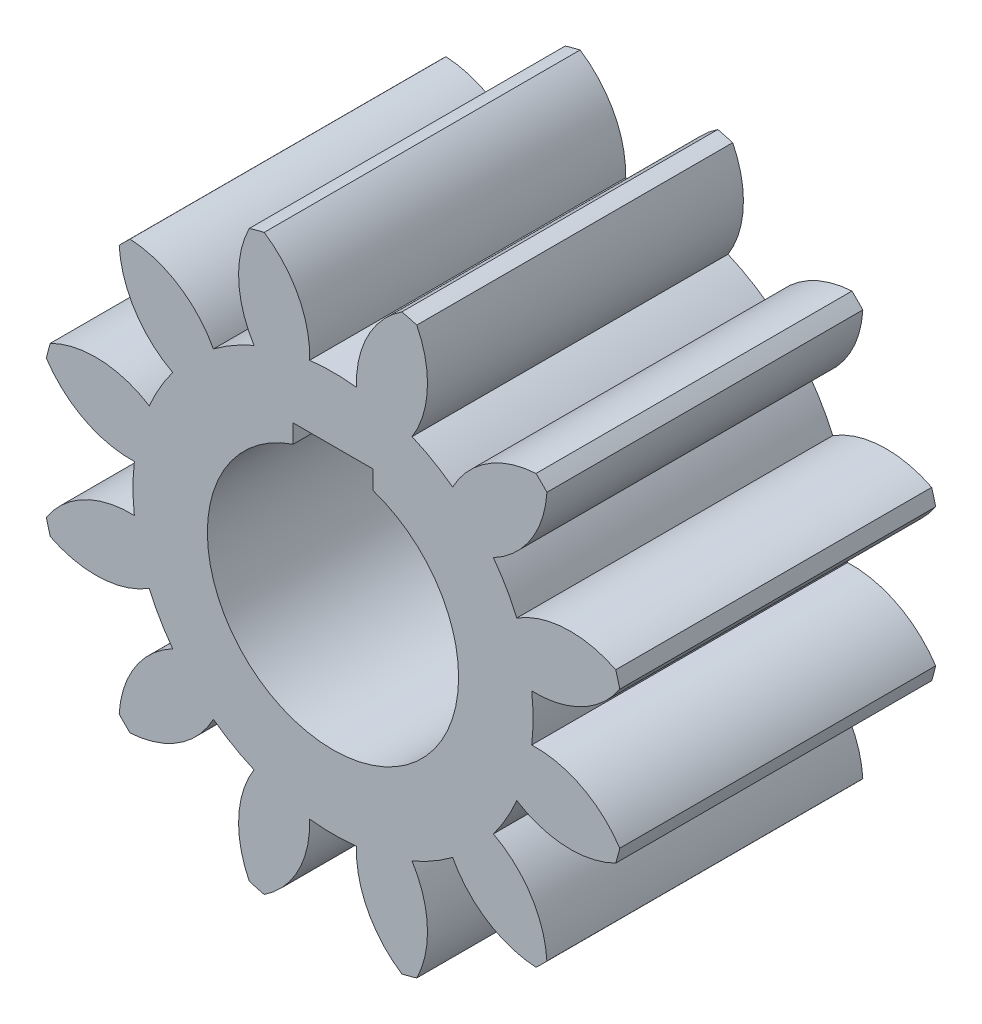
from build123d import *

# Parameters (mm, degrees)
EXTRUDE_1_DEPTH = 15


with BuildPart() as part:
    # 草图2 → 凸台-拉伸1 (new body)
    with BuildSketch(Plane.XY):
        with BuildLine():
            ThreePointArc((-10.154744655, 9.637487276), (-9.402240771, 7.326120193), (-7.613867765, 5.67979037))
            ThreePointArc((-7.613867765, 5.67979037), (-8.226375311, 4.7495), (-8.725776632, 3.753907721))
            ThreePointArc((-8.725776632, 3.753907721), (-11.045726583, 4.479519264), (-13.423681137, 3.975523202))
            ThreePointArc((-13.423681137, 3.975523202), (-13.522961568, 3.623466631), (-13.613010478, 3.268936482))
            ThreePointArc((-13.613010478, 3.268936482), (-11.805639456, 1.643485813), (-9.433698091, 1.111908866))
            ThreePointArc((-9.433698091, 1.111908866), (-9.499, 0), (-9.433698091, -1.111908866))
            ThreePointArc((-9.433698091, -1.111908866), (-11.805639456, -1.643485813), (-13.613010478, -3.268936482))
            ThreePointArc((-13.613010478, -3.268936482), (-13.522961568, -3.623466631), (-13.423681137, -3.975523202))
            ThreePointArc((-13.423681137, -3.975523202), (-11.045726583, -4.479519264), (-8.725776632, -3.753907721))
            ThreePointArc((-8.725776632, -3.753907721), (-8.226375311, -4.7495), (-7.613867765, -5.67979037))
            ThreePointArc((-7.613867765, -5.67979037), (-9.402240771, -7.326120193), (-10.154744655, -9.637487276))
            ThreePointArc((-10.154744655, -9.637487276), (-9.899494937, -9.899494937), (-9.637487276, -10.154744655))
            ThreePointArc((-9.637487276, -10.154744655), (-7.326120193, -9.402240771), (-5.67979037, -7.613867765))
            ThreePointArc((-5.67979037, -7.613867765), (-4.7495, -8.226375311), (-3.753907721, -8.725776632))
            ThreePointArc((-3.753907721, -8.725776632), (-4.479519264, -11.045726583), (-3.975523202, -13.423681137))
            ThreePointArc((-3.975523202, -13.423681137), (-3.623466631, -13.522961568), (-3.268936482, -13.613010478))
            ThreePointArc((-3.268936482, -13.613010478), (-1.643485813, -11.805639456), (-1.111908866, -9.433698091))
            ThreePointArc((-1.111908866, -9.433698091), (0, -9.499), (1.111908866, -9.433698091))
            ThreePointArc((1.111908866, -9.433698091), (1.643485813, -11.805639456), (3.268936482, -13.613010478))
            ThreePointArc((3.268936482, -13.613010478), (3.623466631, -13.522961568), (3.975523202, -13.423681137))
            ThreePointArc((3.975523202, -13.423681137), (4.479519264, -11.045726583), (3.753907721, -8.725776632))
            ThreePointArc((3.753907721, -8.725776632), (4.7495, -8.226375311), (5.67979037, -7.613867765))
            ThreePointArc((5.67979037, -7.613867765), (7.326120193, -9.402240771), (9.637487276, -10.154744655))
            ThreePointArc((9.637487276, -10.154744655), (9.899494937, -9.899494937), (10.154744655, -9.637487276))
            ThreePointArc((10.154744655, -9.637487276), (9.402240771, -7.326120193), (7.613867765, -5.67979037))
            ThreePointArc((7.613867765, -5.67979037), (8.226375311, -4.7495), (8.725776632, -3.753907721))
            ThreePointArc((8.725776632, -3.753907721), (11.045726583, -4.479519264), (13.423681137, -3.975523202))
            ThreePointArc((13.423681137, -3.975523202), (13.522961568, -3.623466631), (13.613010478, -3.268936482))
            ThreePointArc((13.613010478, -3.268936482), (11.805639456, -1.643485813), (9.433698091, -1.111908866))
            ThreePointArc((9.433698091, -1.111908866), (9.499, 0), (9.433698091, 1.111908866))
            ThreePointArc((9.433698091, 1.111908866), (11.805639456, 1.643485813), (13.613010478, 3.268936482))
            ThreePointArc((13.613010478, 3.268936482), (13.522961568, 3.623466631), (13.423681137, 3.975523202))
            ThreePointArc((13.423681137, 3.975523202), (11.045726583, 4.479519264), (8.725776632, 3.753907721))
            ThreePointArc((8.725776632, 3.753907721), (8.226375311, 4.7495), (7.613867765, 5.67979037))
            ThreePointArc((7.613867765, 5.67979037), (9.402240771, 7.326120193), (10.154744655, 9.637487276))
            ThreePointArc((10.154744655, 9.637487276), (9.899494937, 9.899494937), (9.637487276, 10.154744655))
            ThreePointArc((9.637487276, 10.154744655), (7.326120193, 9.402240771), (5.67979037, 7.613867765))
            ThreePointArc((5.67979037, 7.613867765), (4.7495, 8.226375311), (3.753907721, 8.725776632))
            ThreePointArc((3.753907721, 8.725776632), (4.479519264, 11.045726583), (3.975523202, 13.423681137))
            ThreePointArc((3.975523202, 13.423681137), (3.623466631, 13.522961568), (3.268936482, 13.613010478))
            ThreePointArc((3.268936482, 13.613010478), (1.643485813, 11.805639456), (1.111908866, 9.433698091))
            ThreePointArc((1.111908866, 9.433698091), (0, 9.499), (-1.111908866, 9.433698091))
            ThreePointArc((-1.111908866, 9.433698091), (-1.643485813, 11.805639456), (-3.268936482, 13.613010478))
            ThreePointArc((-3.268936482, 13.613010478), (-3.623466631, 13.522961568), (-3.975523202, 13.423681137))
            ThreePointArc((-3.975523202, 13.423681137), (-4.479519264, 11.045726583), (-3.753907721, 8.725776632))
            ThreePointArc((-3.753907721, 8.725776632), (-4.7495, 8.226375311), (-5.67979037, 7.613867765))
            ThreePointArc((-5.67979037, 7.613867765), (-7.326120193, 9.402240771), (-9.637487276, 10.154744655))
            ThreePointArc((-9.637487276, 10.154744655), (-9.899494937, 9.899494937), (-10.154744655, 9.637487276))
        make_face()
        with BuildLine():
            Line((-1.894204479, 6.468399347), (1.888409216, 6.468399347))
            Line((1.888409216, 6.468399347), (1.888409216, 5.589022546))
            ThreePointArc((1.888409216, 5.589022546), (-0.002897631, -6.03248103), (-1.894204479, 5.589022546))
            Line((-1.894204479, 5.589022546), (-1.894204479, 6.468399347))
        make_face(mode=Mode.SUBTRACT)
    extrude(amount=EXTRUDE_1_DEPTH)


solid = part.part
